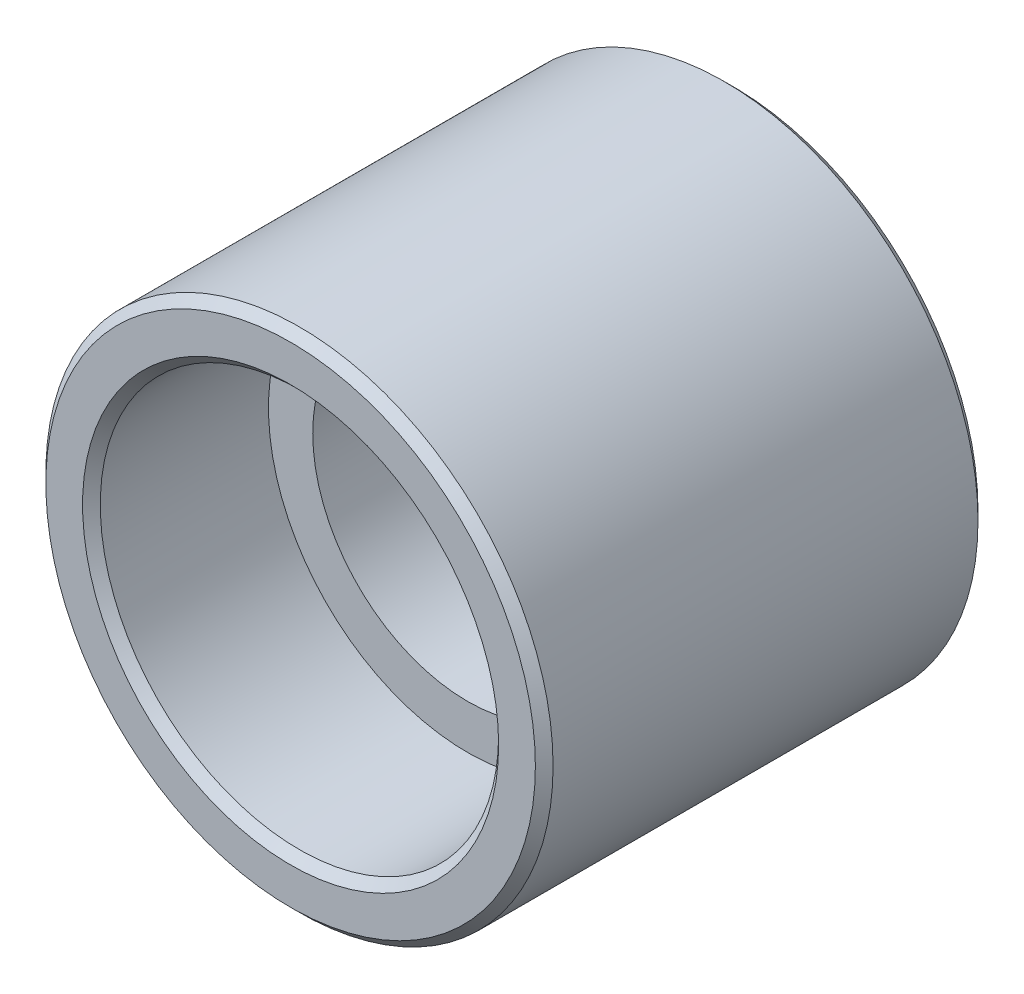
from build123d import *


with BuildPart() as part:
    # Sketch1 → Revolve1 (revolve)
    with BuildSketch(Plane(origin=(0, 0, 0), x_dir=(1, 0, 0), z_dir=(0, 1, 0))):
        Polygon((4.7, 0), (5.53, 0), (5.73, 0.2), (5.73, 9.8), (5.53, 10), (4.7, 10), (4.5, 9.8), (4.5, 6), (3.5, 6), (3.5, 4), (4.5, 4), (4.5, 0.2), align=None)
    revolve(axis=Axis((0, 0, 0), (0, 0, -1)))


solid = part.part
